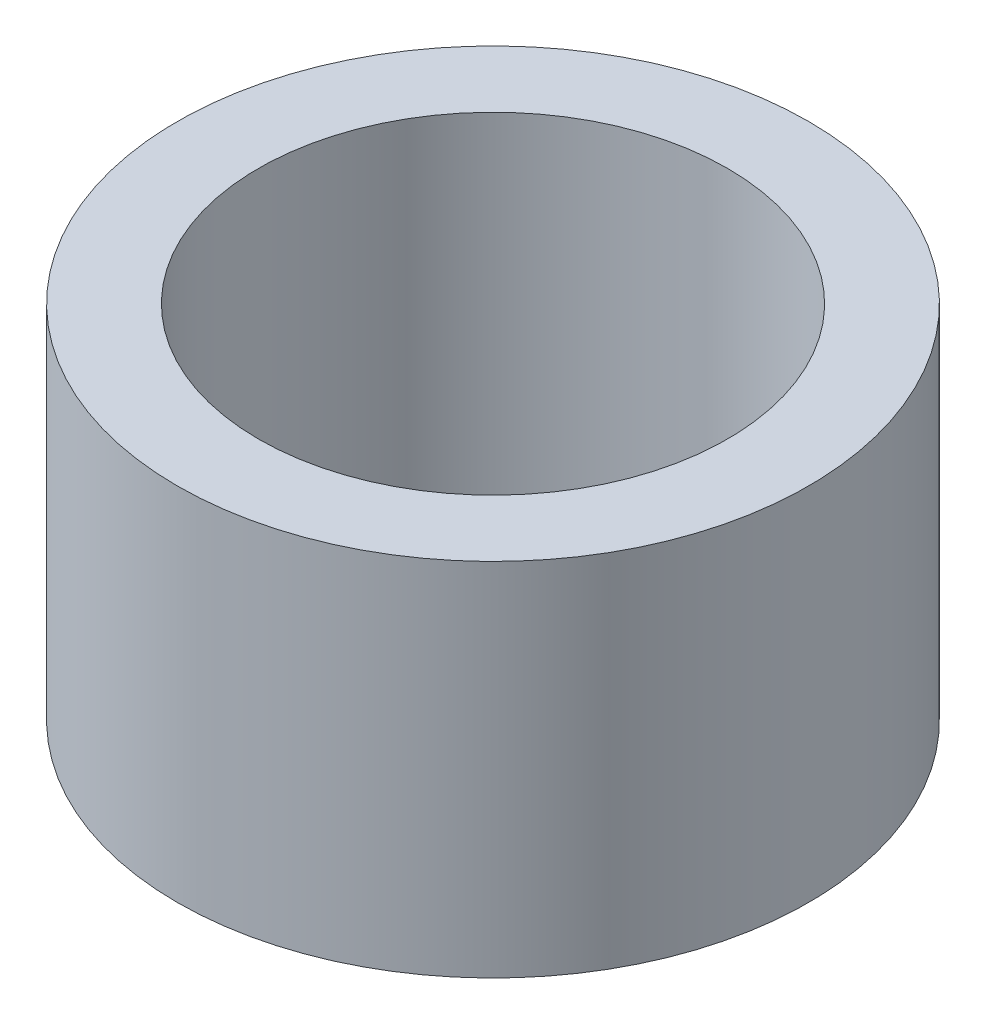
SolidWorks part; units mm, degrees
ref_plane "Front Plane" through (0, 0, 0) normal (0, 0, 1) x (1, 0, 0)
ref_plane "Top Plane" through (0, 0, 0) normal (0, 1, 0) x (1, 0, 0)
ref_plane "Right Plane" through (0, 0, 0) normal (1, 0, 0) x (0, 0, -1)
sketch "Sketch1" plane through (0, 0, 0) normal (0, 0, 1) x (1, 0, 0)
  line L0 (0, 22.6561) -> (0, -16.3439) construction
  line L1 (-17.5, 14.1811) -> (-17.5, -5.8189)
  line L2 (-17.5, -5.8189) -> (-13, -5.8189)
  line L3 (-13, -5.8189) -> (-13, 14.1811)
  line L4 (-13, 14.1811) -> (-17.5, 14.1811)
  dimension "D1" = 4.5
  dimension "D2" = 13
  dimension "D3" = 20
revolve "Revolve1" add sketch "Sketch1" angle 360 about L0
